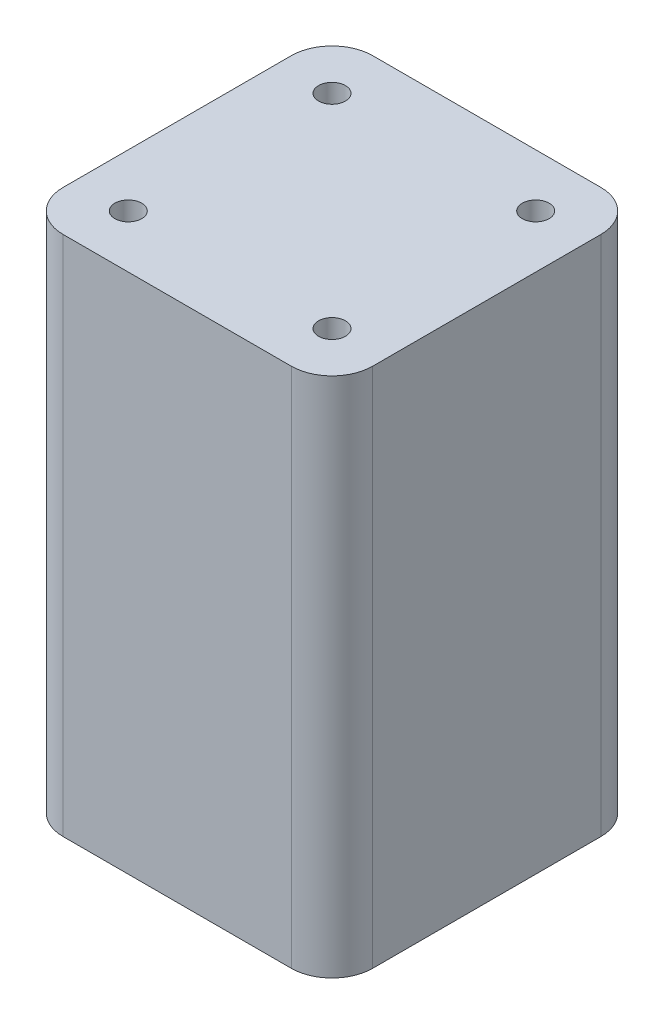
SolidWorks part; units mm, degrees
material "45"
ref_plane "Front Plane" through (0, 0, 0) normal (0, 0, 1) x (1, 0, 0)
ref_plane "Top Plane" through (0, 0, 0) normal (0, 1, 0) x (1, 0, 0)
ref_plane "Right Plane" through (0, 0, 0) normal (1, 0, 0) x (0, 0, -1)
sketch "Sketch1" plane through (0, 0, 0) normal (0, 1, 0) x (1, 0, 0)
  line L1 (-19, 34) -> (19, 34)
  line L2 (-19, 34) -> (-19, -34)
  line L3 (-19, -34) -> (19, -34)
  line L4 (19, 34) -> (19, -34)
  line L5 (-19, 34) -> (19, -34) construction
  line L6 (-19, -34) -> (19, 34) construction
  point P0 (0, 0)
  dimension "D1" = 38
  dimension "D2" = 68
extrude "Boss-Extrude1" add sketch "Sketch1" along normal blind 10
sketch "Sketch2" plane through (0, 10, 0) normal (0, 1, 0) x (1, 0, 0)
  line L0 (19, -34) -> (19, 34) construction
  line L1 (-19, 19) -> (19, 19)
  line L2 (-19, 19) -> (-19, -19)
  line L3 (-19, -19) -> (19, -19)
  line L4 (19, 19) -> (19, -19)
  line L5 (-19, 19) -> (19, -19) construction
  line L6 (-19, -19) -> (19, 19) construction
  point P0 (0, 0)
  dimension "D1" = 38
extrude "Boss-Extrude2" add sketch "Sketch2" along normal blind 54
hole_wizard "M4 Tapped Hole2" positions "Sketch4" profile "Sketch5" tap size "M4" standard "GB"
sketch "Sketch4" plane through (0, 0, 0) normal (0, 1, 0) x (1, 0, 0)
  line L0 (-12.5, 12.5) -> (12.5, 12.5)
  line L1 (12.5, 12.5) -> (12.5, -12.5)
  line L2 (12.5, -12.5) -> (-12.5, -12.5)
  line L3 (-12.5, -12.5) -> (-12.5, 12.5)
  line L5 (0, 12.5) -> (0, 0)
  line L6 (0, 0) -> (-12.5, 0)
  point P0 (-12.5, 12.5)
  point P2 (12.5, 12.5)
  point P4 (-12.5, -12.5)
  point P6 (12.5, -12.5)
  dimension "D1" = 25
  dimension "D2" = 25
sketch "Sketch5" plane through (-12.5, 0, -12.5) normal (1, 0, 0) x (0, 0, -1)
  line L0 (0, 0) -> (0, 11.0914)
  line L1 (0, 11.0914) -> (1.65, 10.1)
  line L2 (1.65, 10.1) -> (1.65, 0)
  line L5 (1.65, 0) -> (0, 0)
  line L10 (0, 11.0914) -> (-1.65, 10.1) construction
  line L11 (0, -6.35) -> (0, 107.95) construction
  dimension "螺纹孔钻头直径" = 3.3
  dimension "螺纹孔钻头深度" = 10.1
  dimension "导头角度" = 118
fillet "Fillet1" radius 5 8 edges at (19, 5, -34) (-19, 5, -34) (19, 37, -19) (-19, 37, -19) (19, 5, 34) (-19, 5, 34) (-19, 37, 19) (19, 37, 19)
hole_wizard "M4 Tapped Hole1" positions "Sketch6" profile "Sketch7" tap size "M4" standard "GB"
sketch "Sketch6" plane through (0, 64, 0) normal (0, 1, 0) x (1, 0, 0)
  line L0 (-12.5, 12.5) -> (-12.5, -12.5)
  line L1 (-12.5, -12.5) -> (12.5, -12.5)
  line L2 (12.5, -12.5) -> (12.5, 12.5)
  line L3 (12.5, 12.5) -> (-12.5, 12.5)
  line L5 (0, 12.5) -> (0, 0)
  line L6 (0, 0) -> (-12.5, 0)
  point P0 (-12.5, 12.5)
  point P2 (12.5, 12.5)
  point P4 (12.5, -12.5)
  point P6 (-12.5, -12.5)
  dimension "D1" = 25
sketch "Sketch7" plane through (-12.5, 64, -12.5) normal (1, 0, 0) x (0, 0, 1)
  line L0 (0, 0) -> (0, 11.0914)
  line L1 (0, 11.0914) -> (1.65, 10.1)
  line L2 (1.65, 10.1) -> (1.65, 0)
  line L5 (1.65, 0) -> (0, 0)
  line L10 (0, 11.0914) -> (-1.65, 10.1) construction
  line L11 (0, -6.35) -> (0, 107.95) construction
  dimension "螺纹孔钻头直径" = 3.3
  dimension "螺纹孔钻头深度" = 10.1
  dimension "导头角度" = 118
cosmetic thread "Hole Thread1" parameters "D1"=8, "D2"=4
cosmetic thread "Hole Thread2" parameters "D1"=8, "D2"=4
cosmetic thread "Hole Thread3" parameters "D1"=8, "D2"=4
cosmetic thread "Hole Thread4" parameters "D1"=8, "D2"=4
sketch "Sketch8" plane through (0, 64, 0) normal (0, 1, 0) x (1, 0, 0)
  line L0 (-14, -19) -> (14, -19) construction
  line L1 (-14, 19) -> (14, 19)
  line L2 (-19, 14) -> (-19, -14)
  line L3 (-14, -19) -> (14, -19)
  line L4 (19, 14) -> (19, -14)
  line L5 (-19, 19) -> (19, -19) construction
  line L6 (-19, -19) -> (19, 19) construction
  arc A0 (14, 19) -> (19, 14) centre (14, 14) cw
  arc A1 (-14, 19) -> (-19, 14) centre (-14, 14) ccw
  arc A2 (-19, -14) -> (-14, -19) centre (-14, -14) ccw
  arc A3 (14, -19) -> (19, -14) centre (14, -14) ccw
  point P0 (0, 0)
  dimension "D1" = 5
extrude "Cut-Extrude1" cut sketch "Sketch8" against normal through all flip side to cut
